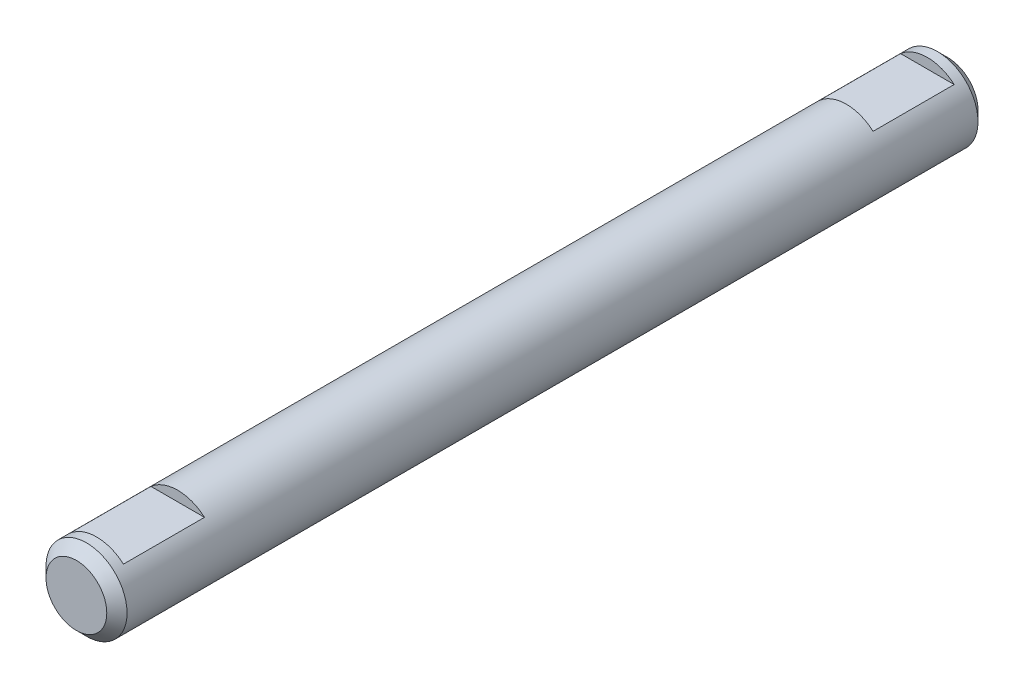
from build123d import *

# Parameters (mm, degrees)
SKETCH1_R           = 2
BOSS_EXTRUDE1_DEPTH = 21.5
SKETCH2_W           = 15.41853157
SKETCH2_H           = 4
SKETCH2_W_2         = 11.817796653
CUT_EXTRUDE1_DEPTH  = 0.5
CHAMFER1_SIZE       = 0.5


with BuildPart() as part:
    # Sketch1 → Boss-Extrude1 (new, symmetric)
    with BuildSketch(Plane.XY):
        Circle(SKETCH1_R)
    extrude(amount=BOSS_EXTRUDE1_DEPTH, both=True)

    # Sketch2 → Cut-Extrude1 (cut)
    with BuildSketch(Plane(origin=(0, 2, 0), x_dir=(-1, 0, 0), z_dir=(0, 1, 0))):
        with Locations((0, 18.5)):
            Rectangle(SKETCH2_W, SKETCH2_H)
        with Locations((0.877102096, -18.5)):
            Rectangle(SKETCH2_W_2, SKETCH2_H)
    extrude(amount=-CUT_EXTRUDE1_DEPTH, mode=Mode.SUBTRACT)

    # Chamfer1
    chamfer1_edges = [part.edges().sort_by_distance(p)[0] for p in [
        (-2, 0, -21.5),
        (-2, 0, 21.5),
    ]]
    chamfer(chamfer1_edges, length=CHAMFER1_SIZE)


solid = part.part
